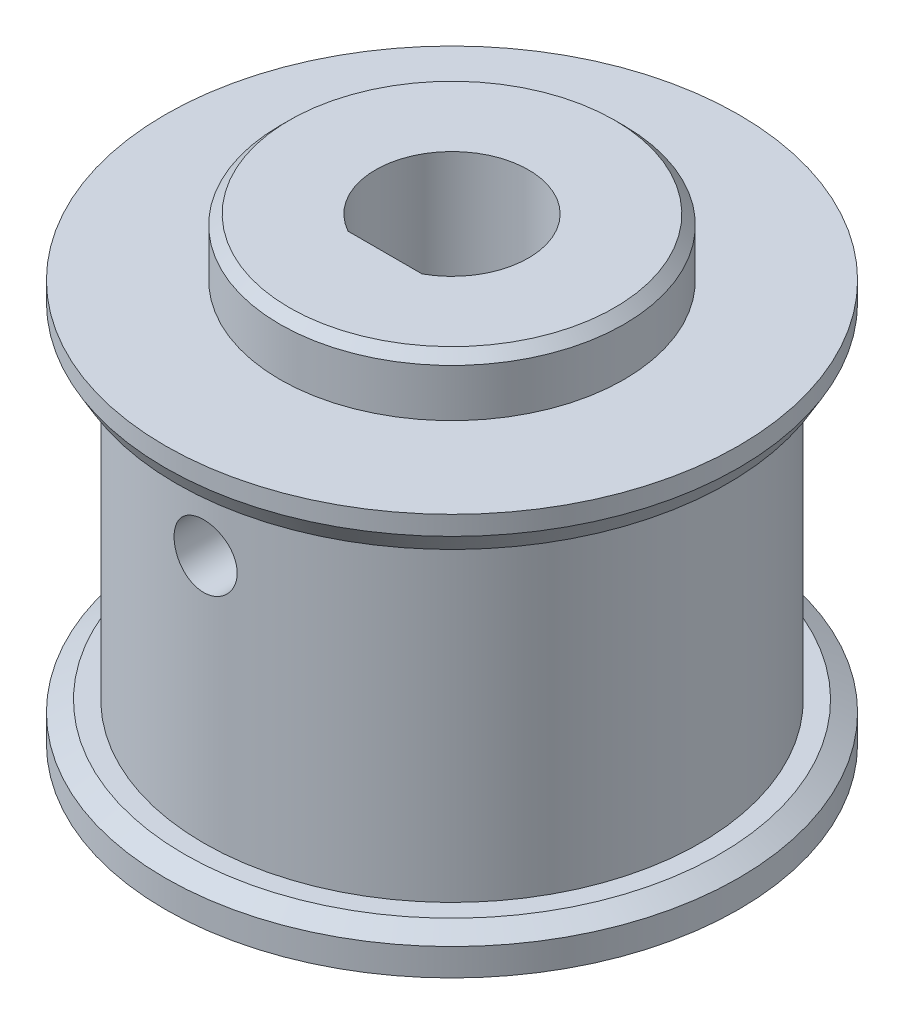
from build123d import *

# Parameters (mm, degrees)
SKETCH_5_R               = 20.566311538
CUT_EXTRUDE_1_DEPTH      = 0.5
SKETCH_6_R               = 21.52826295
CUT_EXTRUDE_2_DEPTH      = 0.5
EXTRUDE_START            = 11
SKETCH_7_R               = 8.5
SKETCH_7_R_2             = 4
EXTRUDE_1_DEPTH          = 11
SKETCH_10_R              = 15
CUT_EXTRUDE_3_DEPTH      = 15
SKETCH_11_R              = 15
SKETCH_11_R_2            = 4
EXTRUDE_2_DEPTH          = 0.5
EXTRUDE_START_2          = 0.5
SKETCH_12_R              = 15
SKETCH_12_R_2            = 4
EXTRUDE_3_DEPTH          = 0.5
EXTRUDE_START_3          = 8
SKETCH_14_R              = 7
SKETCH_14_R_2            = 4
EXTRUDE_5_DEPTH          = 8
SKETCH_17_R              = 17.215216586
CUT_EXTRUDE_4_DEPTH      = 30.849623113
SKETCH_18_R              = 9
SKETCH_18_R_2            = 4
EXTRUDE_6_DEPTH          = 8
CHAMFER_1_SIZE           = 1
CHAMFER_1_SIZE2          = 0.577350269
CHAMFER_2_SIZE           = 1
CHAMFER_2_SIZE2          = 0.577350269
CHAMFER_3_SIZE           = 0.5
SKETCH_22_R              = 10.406041916
CUT_EXTRUDE_6_DEPTH      = 5
SKETCH_24_W              = 7.050057501
SKETCH_24_H              = 1.266031453
EXTRUDE_7_DEPTH          = 24
SKETCH_19_W              = 1.65
SKETCH_19_H              = 15
PATTERN_CIRCULAR_1_COUNT = 2
PATTERN_CIRCULAR_1_ANGLE = 90
CHAMFER_4_SIZE           = 0.5


with BuildPart() as part:
    # 草图1 → 旋转1 (revolve)
    with BuildSketch(Plane.XY, mode=Mode.PRIVATE) as revolve_1_sk:
        Polygon((4, 0), (4, 21), (15, 21), (15, 19), (12.99, 19), (12.99, 2), (15, 2), (15, 0), align=None)
    revolve(revolve_1_sk.sketch.rotate(Axis((0, 0, 0), (0, 1, 0)), 90), axis=Axis((0, 0, 0), (0, 1, 0)))

    # 草图5 → 切除-拉伸1 (cut)
    with BuildSketch(Plane.XZ):
        Circle(SKETCH_5_R)
    extrude(amount=-CUT_EXTRUDE_1_DEPTH, mode=Mode.SUBTRACT)

    # 草图6 → 切除-拉伸2 (cut)
    with BuildSketch(Plane(origin=(0, 21, 0), x_dir=(1, 0, 0), z_dir=(0, 1, 0))):
        Circle(SKETCH_6_R)
    extrude(amount=-CUT_EXTRUDE_2_DEPTH, mode=Mode.SUBTRACT)

    # 草图7 → 凸台-拉伸1 (add)
    with BuildSketch(Plane(origin=(0, 20.5, 0), x_dir=(1, 0, 0), z_dir=(0, 1, 0)).offset(EXTRUDE_START)):
        with Locations(Location((0, 0, 0), (0, 0, 270))):
            Circle(SKETCH_7_R)
        with Locations(Location((0, 0, 0), (0, 0, 90))):
            Circle(SKETCH_7_R_2, mode=Mode.SUBTRACT)
    extrude(amount=-EXTRUDE_1_DEPTH)

    # 草图10 → 切除-拉伸3 (cut)
    with BuildSketch(Plane(origin=(0, 20.5, 0), x_dir=(1, 0, 0), z_dir=(0, 1, 0))):
        with Locations(Location((0, 0, 0), (0, 0, 90))):
            Circle(SKETCH_10_R)
    extrude(amount=CUT_EXTRUDE_3_DEPTH, mode=Mode.SUBTRACT)

    # 草图11 → 凸台-拉伸2 (add)
    with BuildSketch(Plane(origin=(0, 20.5, 0), x_dir=(1, 0, 0), z_dir=(0, 1, 0))):
        with Locations(Location((0, 0, 0), (0, 0, 90))):
            Circle(SKETCH_11_R)
        with Locations(Location((0, 0, 0), (0, 0, 90))):
            Circle(SKETCH_11_R_2, mode=Mode.SUBTRACT)
    extrude(amount=EXTRUDE_2_DEPTH)

    # 草图12 → 凸台-拉伸3 (add)
    with BuildSketch(Plane.XZ.offset(-0.5).offset(EXTRUDE_START_2)):
        with Locations(Location((0, 0, 0), (0, 0, 270))):
            Circle(SKETCH_12_R)
        with Locations(Location((0, 0, 0), (0, 0, 270))):
            Circle(SKETCH_12_R_2, mode=Mode.SUBTRACT)
    extrude(amount=-EXTRUDE_3_DEPTH)

    # 草图14 → 凸台-拉伸5 (add)
    with BuildSketch(Plane(origin=(0, 21, 0), x_dir=(1, 0, 0), z_dir=(0, 1, 0)).offset(EXTRUDE_START_3)):
        with Locations(Location((0, 0, 0), (0, 0, 270))):
            Circle(SKETCH_14_R)
        with Locations(Location((0, 0, 0), (0, 0, 90))):
            Circle(SKETCH_14_R_2, mode=Mode.SUBTRACT)
    extrude(amount=-EXTRUDE_5_DEPTH)

    # 草图17 → 切除-拉伸4 (cut, through all)
    with BuildSketch(Plane(origin=(0, 21, 0), x_dir=(1, 0, 0), z_dir=(0, 1, 0))):
        Circle(SKETCH_17_R)
    extrude(amount=CUT_EXTRUDE_4_DEPTH, mode=Mode.SUBTRACT)

    # 草图18 → 凸台-拉伸6 (add)
    with BuildSketch(Plane(origin=(0, 21, 0), x_dir=(1, 0, 0), z_dir=(0, 1, 0)).offset(EXTRUDE_START_3)):
        with Locations(Location((0, 0, 0), (0, 0, 270))):
            Circle(SKETCH_18_R)
        with Locations(Location((0, 0, 0), (0, 0, 90))):
            Circle(SKETCH_18_R_2, mode=Mode.SUBTRACT)
    extrude(amount=-EXTRUDE_6_DEPTH)

    # 倒角1
    chamfer_1_edges = [part.edges().sort_by_distance(p)[0] for p in [
        (0, 19, 15),
    ]]
    chamfer_1_side = [part.faces().sort_by_distance(p)[0] for p in [
        (0, 20, 15),
    ]]
    chamfer(chamfer_1_edges, length=CHAMFER_1_SIZE, length2=CHAMFER_1_SIZE2, reference=chamfer_1_side[0])

    # 倒角2
    chamfer_2_edges = [part.edges().sort_by_distance(p)[0] for p in [
        (0, 2, 15),
    ]]
    chamfer_2_side = [part.faces().sort_by_distance(p)[0] for p in [
        (0, 2, 13.414264069),
    ]]
    chamfer(chamfer_2_edges, length=CHAMFER_2_SIZE, length2=CHAMFER_2_SIZE2, reference=chamfer_2_side[0])

    # 倒角3
    chamfer_3_edges = [part.edges().sort_by_distance(p)[0] for p in [
        (0, 29, -9),
    ]]
    chamfer(chamfer_3_edges, length=CHAMFER_3_SIZE)

    # 草图22 → 切除-拉伸6 (cut)
    with BuildSketch(Plane(origin=(0, 29, 0), x_dir=(1, 0, 0), z_dir=(0, 1, 0))):
        Circle(SKETCH_22_R)
    extrude(amount=-CUT_EXTRUDE_6_DEPTH, mode=Mode.SUBTRACT)

    # 草图24 → 凸台-拉伸7 (add)
    with BuildSketch(Plane.XZ):
        with Locations((0.325970853, 4.133015727)):
            Rectangle(SKETCH_24_W, SKETCH_24_H)
    extrude(amount=-EXTRUDE_7_DEPTH)

    # 草图19 → M4 螺纹孔1 (revolve, cut)
    with BuildSketch(Plane(origin=(0, 15, 0), x_dir=(0, 1, 0), z_dir=(1, 0, 0))):
        with Locations((0.825, 7.5)):
            Rectangle(SKETCH_19_W, SKETCH_19_H)
    hole_wizard_m4_1 = revolve(axis=Axis((0, 15, -6.35), (0, 0, 1)), mode=Mode.SUBTRACT)

    # 阵列(圆周)1: M4 螺纹孔1 ×2 about axis
    pattern_circular_1_axis = Axis((0, 0, 0), (0, -1, 0))
    for i in range(1, PATTERN_CIRCULAR_1_COUNT):
        add(hole_wizard_m4_1.rotate(pattern_circular_1_axis, i * PATTERN_CIRCULAR_1_ANGLE / (PATTERN_CIRCULAR_1_COUNT - 1)), mode=Mode.SUBTRACT)

    # 倒角4
    chamfer_4_edges = [part.edges().sort_by_distance(p)[0] for p in [
        (0, 24, -9),
    ]]
    chamfer(chamfer_4_edges, length=CHAMFER_4_SIZE)


solid = part.part
